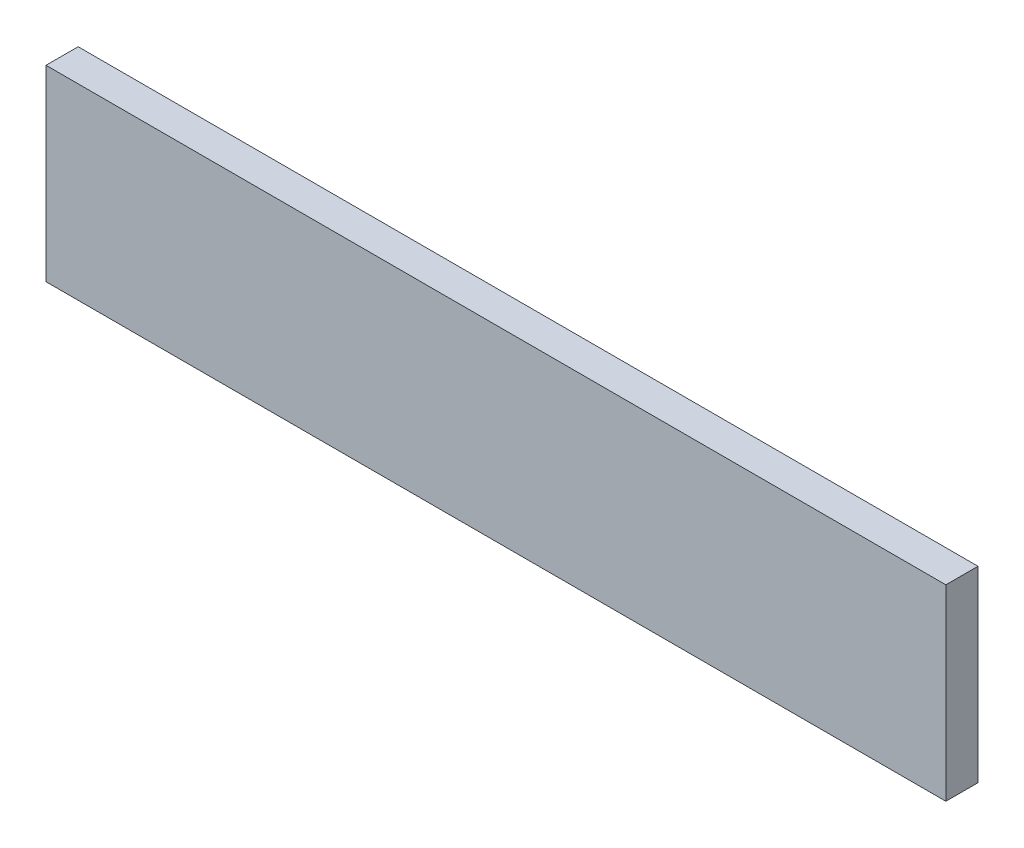
from build123d import *

# Parameters (mm, degrees)
SKETCH1_W           = 840
SKETCH1_H           = 175
BOSS_EXTRUDE1_DEPTH = 30


with BuildPart() as part:
    # Sketch1 → Boss-Extrude1 (new body)
    with BuildSketch(Plane.XY):
        with Locations((420, 87.5)):
            Rectangle(SKETCH1_W, SKETCH1_H)
    extrude(amount=BOSS_EXTRUDE1_DEPTH)


solid = part.part
